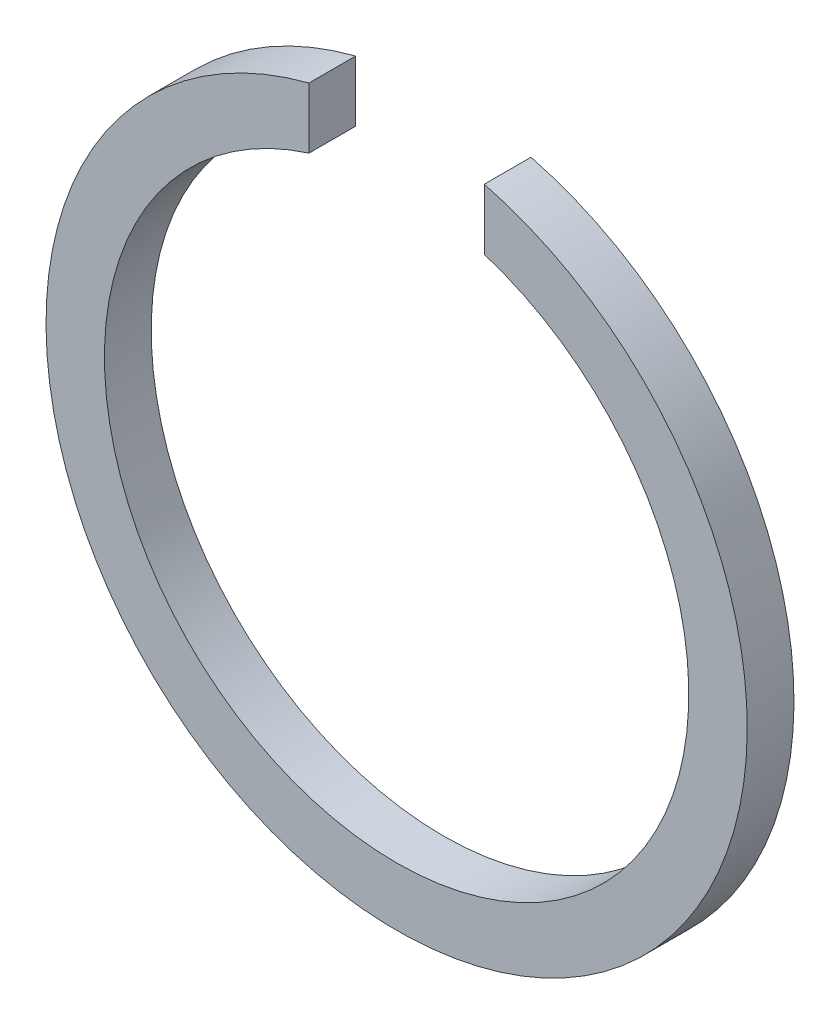
SolidWorks part; units mm, degrees
ref_plane "Front Plane" through (0, 0, 0) normal (0, 0, 1) x (1, 0, 0)
ref_plane "Top Plane" through (0, 0, 0) normal (0, 1, 0) x (1, 0, 0)
ref_plane "Right Plane" through (0, 0, 0) normal (1, 0, 0) x (0, 0, -1)
sketch "Sketch1" plane through (0, 0, 0) normal (0, 0, 1) x (1, 0, 0)
  circle A0 centre (0, 0) radius 60
  circle A1 centre (0, 0) radius 50
  dimension "D1" = 120
  dimension "D2" = 100
extrude "Boss-Extrude1" add sketch "Sketch1" along normal blind 8
sketch "Sketch2" plane through (0, 0, 8) normal (0, 0, 1) x (1, 0, 0)
  line L1 (-15, 15.58) -> (15, 15.58)
  line L2 (-15, 15.58) -> (-15, 87.4146)
  line L3 (-15, 87.4146) -> (15, 87.4146)
  line L4 (15, 15.58) -> (15, 87.4146)
  line L5 (-15, 15.58) -> (15, 87.4146) construction
  line L6 (-15, 87.4146) -> (15, 15.58) construction
  point P0 (0, 51.4973)
  dimension "D1" = 30
extrude "Cut-Extrude1" cut sketch "Sketch2" against normal blind 15
